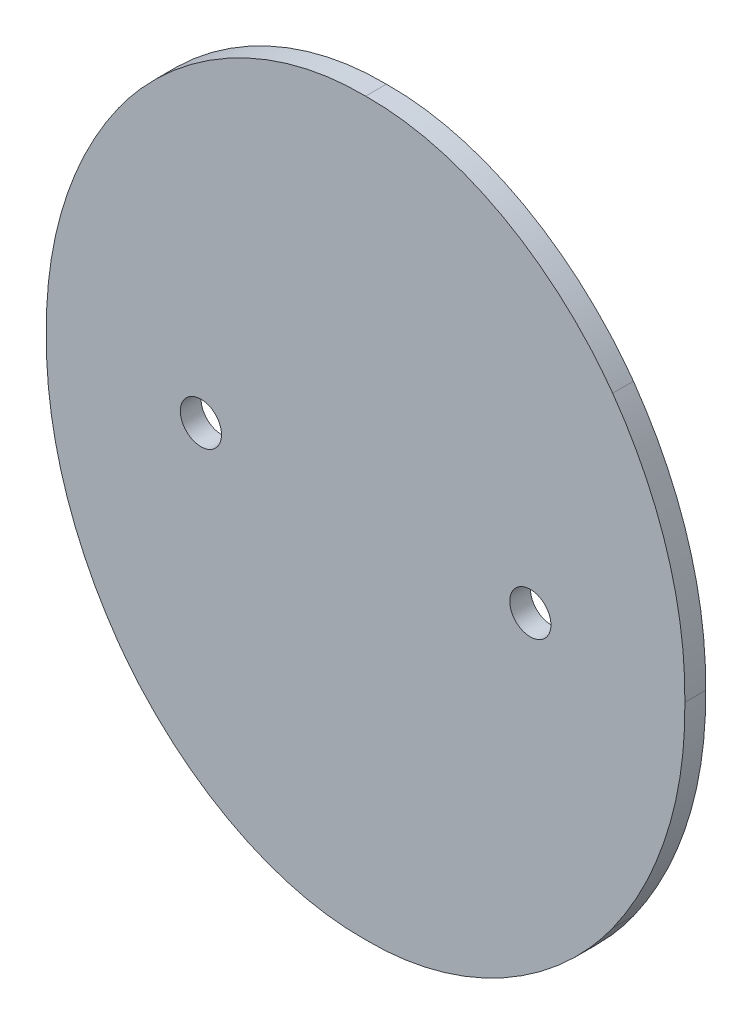
from build123d import *

# Parameters (mm, degrees)
BOSS_EXTRUDE1_DEPTH = 1.6002
SKETCH2_R           = 1.5875
CUT_EXTRUDE1_DEPTH  = 1.6002


with BuildPart() as part:
    # Sketch1 → Boss-Extrude1 (new body)
    with BuildSketch(Plane.XY):
        with BuildLine():
            add(Edge.make_bspline(
                [(0, -28.1686), (-7.577848525, -28.285084622), (-14.719054348, -23.91013337), (-19.05, -17.8562)],
                knots=[0, 0, 0, 0, 1, 1, 1, 1], degree=3))
            ThreePointArc((-19.05, -17.8562), (-23.254686005, -9.371516124), (-24.6126, 0))
            ThreePointArc((-24.6126, 0), (-23.254686005, 9.371516124), (-19.05, 17.8562))
            add(Edge.make_bspline(
                [(0, 28.1686), (-7.577848525, 28.285084622), (-14.719054348, 23.91013337), (-19.05, 17.8562)],
                knots=[0, 0, 0, 0, 1, 1, 1, 1], degree=3))
            add(Edge.make_bspline(
                [(0, 28.1686), (7.577848525, 28.285084622), (14.719054348, 23.91013337), (19.05, 17.8562)],
                knots=[0, 0, 0, 0, 1, 1, 1, 1], degree=3))
            ThreePointArc((19.05, 17.8562), (23.254686005, 9.371516124), (24.6126, 0))
            ThreePointArc((24.6126, 0), (23.254686005, -9.371516124), (19.05, -17.8562))
            add(Edge.make_bspline(
                [(0, -28.1686), (7.577848525, -28.285084622), (14.719054348, -23.91013337), (19.05, -17.8562)],
                knots=[0, 0, 0, 0, 1, 1, 1, 1], degree=3))
        make_face()
    extrude(amount=BOSS_EXTRUDE1_DEPTH)

    # Sketch2 → Cut-Extrude1 (cut)
    with BuildSketch(Plane.XY.offset(1.6002)):
        with Locations((-12.7, 0)):
            Circle(SKETCH2_R)
        with Locations((12.7, 0)):
            Circle(SKETCH2_R)
    extrude(amount=-CUT_EXTRUDE1_DEPTH, mode=Mode.SUBTRACT)


solid = part.part
